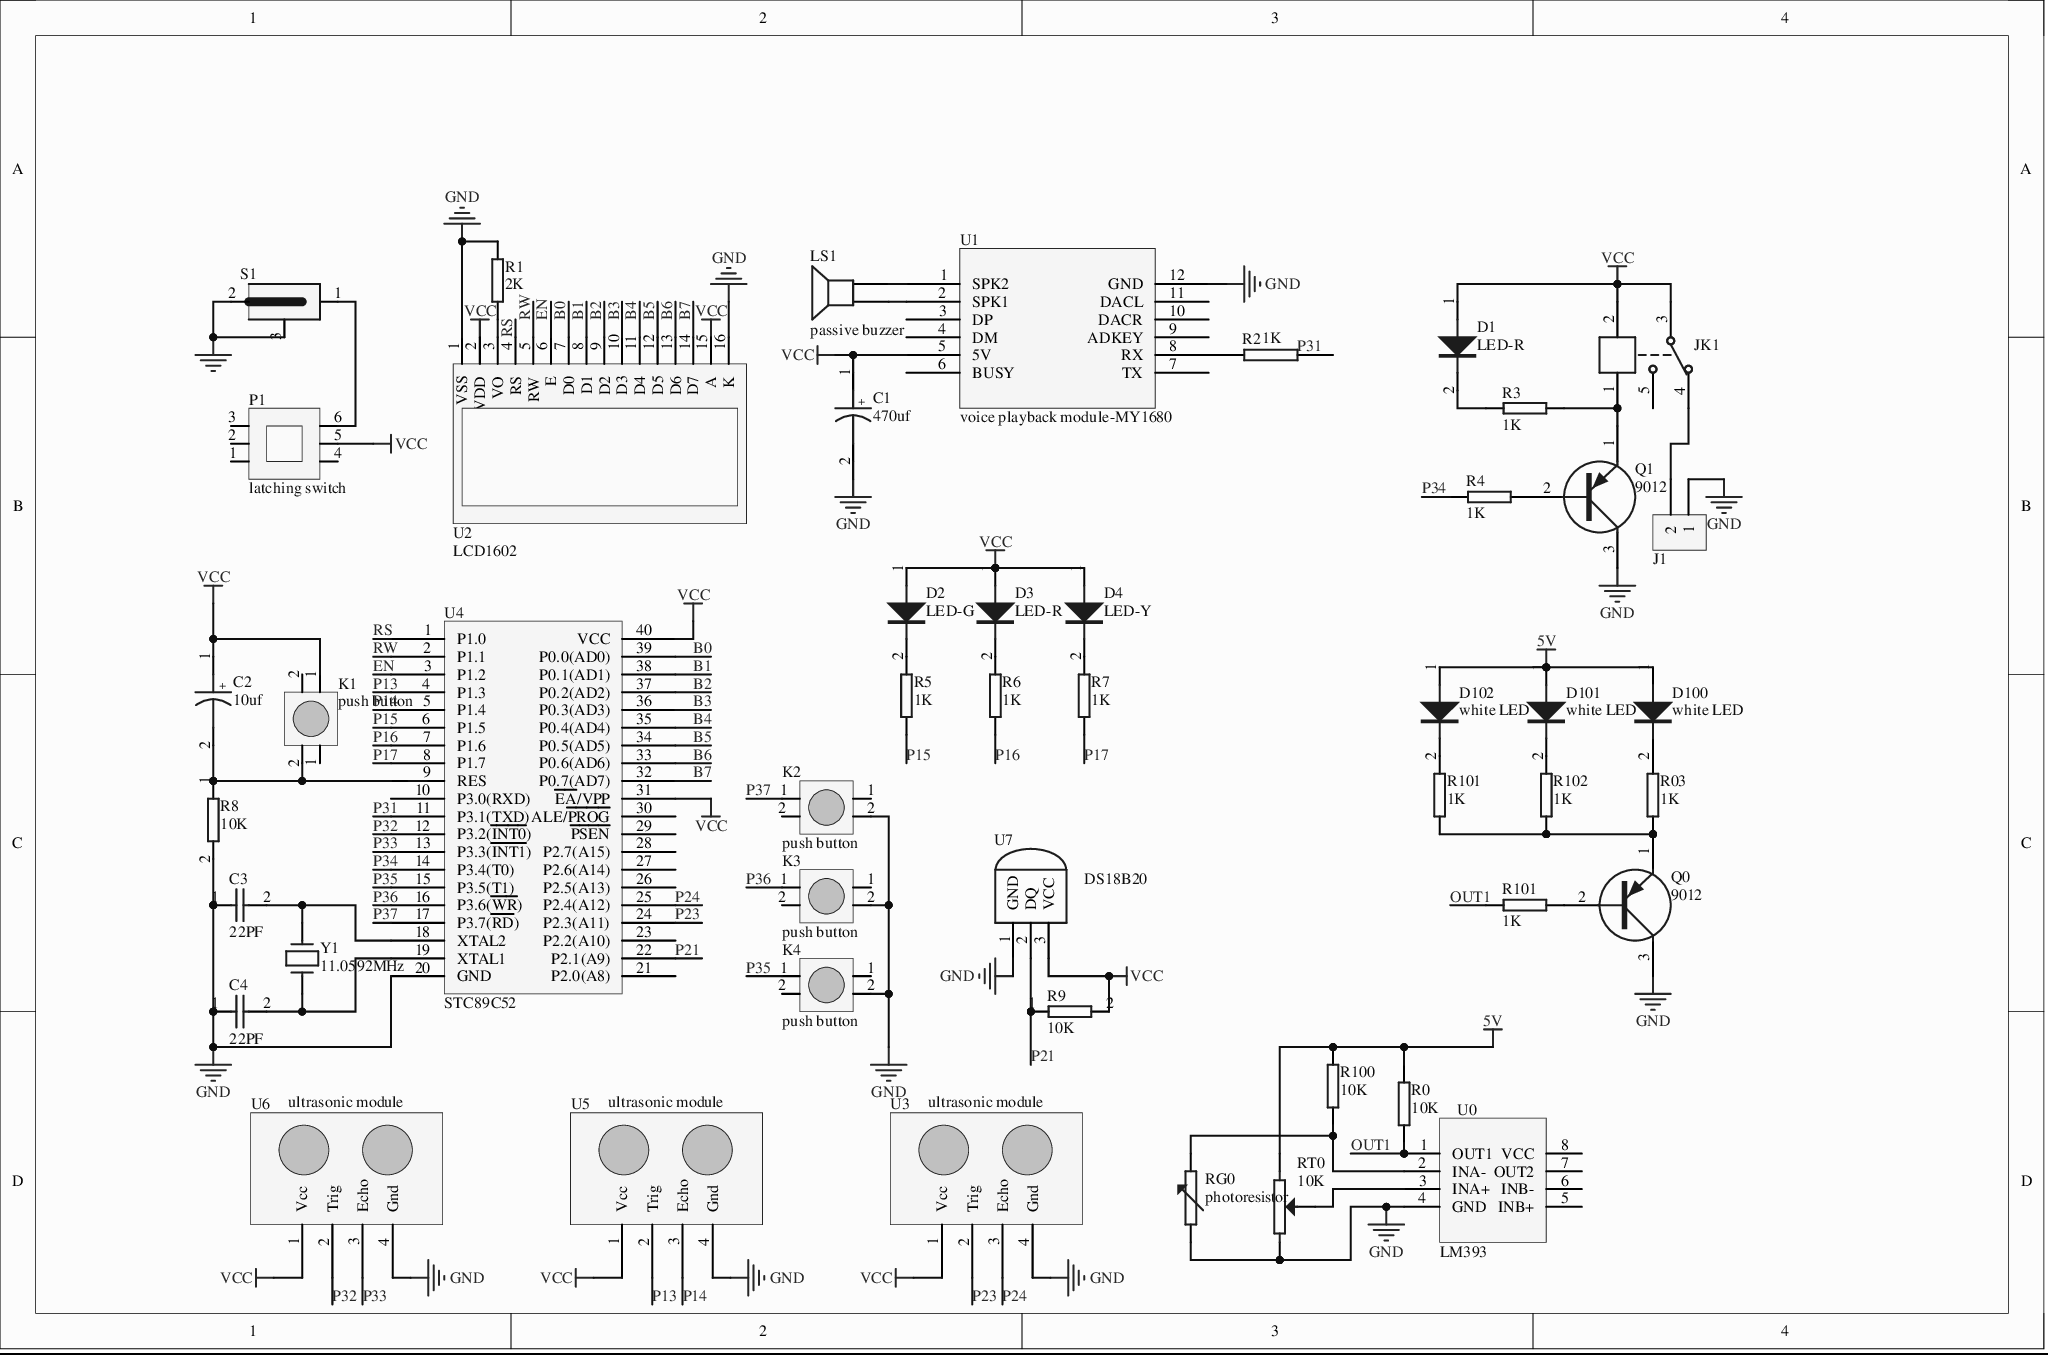
[diagram p0: MISC80724-9.SchDoc]
# Altium project MISC80724-7.PrjPcb
1 sheet, 48 parts. Net scope: global (net labels, ports and power ports of the same name join across sheets).
Board file: MISC80724.PcbDoc

## Sheet MISC80724-9.SchDoc
size A4

### Parts
(Parts that share a designator on the sheet are numbered #1, #2 ... from top to bottom, then left to right.)
C1  470uf  [RB7.6-15]
C2  10uf  [RB7.6-15]
C3  22PF  [RAD-0.3]
C4  22PF  [RAD-0.3]
D1  LED-R  [LED]
D2  LED-G  [LED]
D3  LED-R  [LED]
D4  LED-Y  [LED]
D100  white LED  [LED]
D101  white LED  [LED]
D102  white LED  [LED]
J1  (no value)  [KF301-5.0-2P]
JK1  HFKW-012-1ZW  [012-1ZW_W]  (value not drawn)
K1  push button  [四脚轻触开关]
K2  push button  [四脚轻触开关]
K3  push button  [四脚轻触开关]
K4  push button  [四脚轻触开关]
LS1  passive buzzer  [PIN2]
P1  latching switch  [自锁开关]
Q0  9012  [TO-92A]
Q1  9012  [TO-92A]
R0  10K  [AXIAL-0.4]
R1  2K  [AXIAL-0.4]
R2  1K  [AXIAL-0.4]
R3  1K  [AXIAL-0.4]
R03  1K  [AXIAL-0.4]
R4  1K  [AXIAL-0.4]
R5  1K  [AXIAL-0.4]
R6  1K  [AXIAL-0.4]
R7  1K  [AXIAL-0.4]
R8  10K  [AXIAL-0.4]
R9  10K  [AXIAL-0.4]
R100  10K  [AXIAL-0.4]
R101#1  1K  [AXIAL-0.4]
R101#2  1K  [AXIAL-0.4]
R102  1K  [AXIAL-0.4]
RG0  photoresistor  [AXIAL-0.6]
RT0  10K  [电位器]
S1  (no value)  [KLD-0202]
U0  LM393  [DIP-8]
U1  voice playback module-MY1680  [MY1680]
U2  LCD1602  [LCD1602]
U3  ultrasonic module  [HDR1X4]
U4  STC89C52  [DIP-40]
U5  ultrasonic module  [HDR1X4]
U6  ultrasonic module  [HDR1X4]
U7  DS18B20  [DS18B20]
Y1  11.0592MHz  [XTAL_US]

### Nets
5V: D100.1 D101.1 D102.1 R0.2 R100.2 RT0.1
GND: C1.2 C3.1 C4.1 J1.1 K2.2 K3.2 K4.2 Q0.3(C) Q1.3(C) R1.2 R8.2 RG0.1 RT0.2 S1.2 S1.3 U0.4(GND) U1.12(GND) U2.1(VSS) U2.16(K) U3.4(Gnd) U4.20(GND) U5.4(Gnd) U6.4(Gnd) U7.1(GND)
VCC: C1.1 C2.1 D1.1 D2.1 D3.1 D4.1 JK1.2 JK1.3 K1.1 P1.5 R9.2 U1.5(5V) U2.2(VDD) U2.15(A) U3.1(Vcc) U4.31(~{EA}/VPP) U4.40(VCC) U5.1(Vcc) U6.1(Vcc) U7.3(VCC)
B0: U2.7(D0) U4.39(P0.0(AD0))
B1: U2.8(D1) U4.38(P0.1(AD1))
B2: U2.9(D2) U4.37(P0.2(AD2))
B3: U2.10(D3) U4.36(P0.3(AD3))
B4: U2.11(D4) U4.35(P0.4(AD4))
B5: U2.12(D5) U4.34(P0.5(AD5))
B6: U2.13(D6) U4.33(P0.6(AD6))
B7: U2.14(D7) U4.32(P0.7(AD7))
EN: U2.6(E) U4.3(P1.2)
OUT1: R0.1 R101#2.2 U0.1(OUT1)
P13: U4.4(P1.3) U5.2(Trig)
P14: U4.5(P1.4) U5.3(Echo)
P15: R5.1 U4.6(P1.5)
P16: R6.1 U4.7(P1.6)
P17: R7.1 U4.8(P1.7)
P21: R9.1 U4.22(P2.1(A9)) U7.2(DQ)
P23: U3.2(Trig) U4.24(P2.3(A11))
P24: U3.3(Echo) U4.25(P2.4(A12))
P31: U4.11(P3.1(TXD))
P32: U4.12(P3.2(~{INT0})) U6.2(Trig)
P33: U4.13(P3.3(~{INT1})) U6.3(Echo)
P34: R4.1 U4.14(P3.4(T0))
P35: K4.1 U4.15(P3.5(T1))
P36: K3.1 U4.16(P3.6(~{WR}))
P37: K2.1 U4.17(P3.7(~{RD}))
RS: U2.4(RS) U4.1(P1.0)
RW: U2.5(RW) U4.2(P1.1)
NetC2_2: C2.2 K1.2 R8.1 U4.9(RES)
NetC3_2: C3.2 U4.18(XTAL2) Y1.1
NetC4_2: C4.2 U4.19(XTAL1) Y1.2
NetD1_2: D1.2 R3.1
NetD2_2: D2.2 R5.2
NetD3_2: D3.2 R6.2
NetD4_2: D4.2 R7.2
NetD100_2: D100.2 R03.2
NetD101_2: D101.2 R102.2
NetD102_2: D102.2 R101#1.2
NetJ1_2: J1.2 JK1.4
NetJK1_1: JK1.1 Q1.1(E) R3.2
NetLS1_1: LS1.1 U1.2(SPK1)
NetLS1_2: LS1.2 U1.1(SPK2)
NetP1_6: P1.6 S1.1
NetQ0_1: Q0.1(E) R03.1 R101#1.1 R102.1
NetQ0_2: Q0.2(B) R101#2.1
NetQ1_2: Q1.2(B) R4.2
NetR1_1: R1.1 U2.3(VO)
NetR2_1: R2.1 U1.8(RX)
NetR100_1: R100.1 RG0.2 U0.2(INA-)
NetRT0_3: RT0.3(W) U0.3(INA+)

Not connected (* = marked no-connect by the designer): JK1 5; P1 1 2 3 4; R2 2; U0 5(INB+) 6(INB-) 7(OUT2) 8(VCC); U1 3(DP) 4(DM) 6(BUSY) 7(TX) 9(ADKEY) 10(DACR) 11(DACL); U4 10(P3.0(RXD)) 21(P2.0(A8)) 23(P2.2(A10)) 26(P2.5(A13)) 27(P2.6(A14)) 28(P2.7(A15)) 29(~{PSEN}) 30(ALE/~{PROG})

### Notes on the sheet
- Labels drawn without touching a wire or pin: P31

### Library data of the parts
C1 C2 = 电解电容
C3 C4 = 瓷片电容
D1-D4 D100-D102 = LED-5MM
J1 = 端子2P-5mm
JK1 = HFKW-012-1ZW: 12V one-group changeover; BOM名称: BOM name 12V relay; 版权归属: Copyright owner COMPANY_A
K1-K4 = 按键
LS1 = SPEAKER
P1 = 自锁开关
Q0 Q1 = PNP三极管
R0 R1 R3 R03-R9 R100 R101#1 R101#2 R102 = 电阻-定值
R2 = RES2
RG0 = 电阻-光敏
RT0 = 电位器
S1 = 电源接口-小
U1 = Component_1
U3 U5 U6 = 超声波模块
Y1 = 晶振